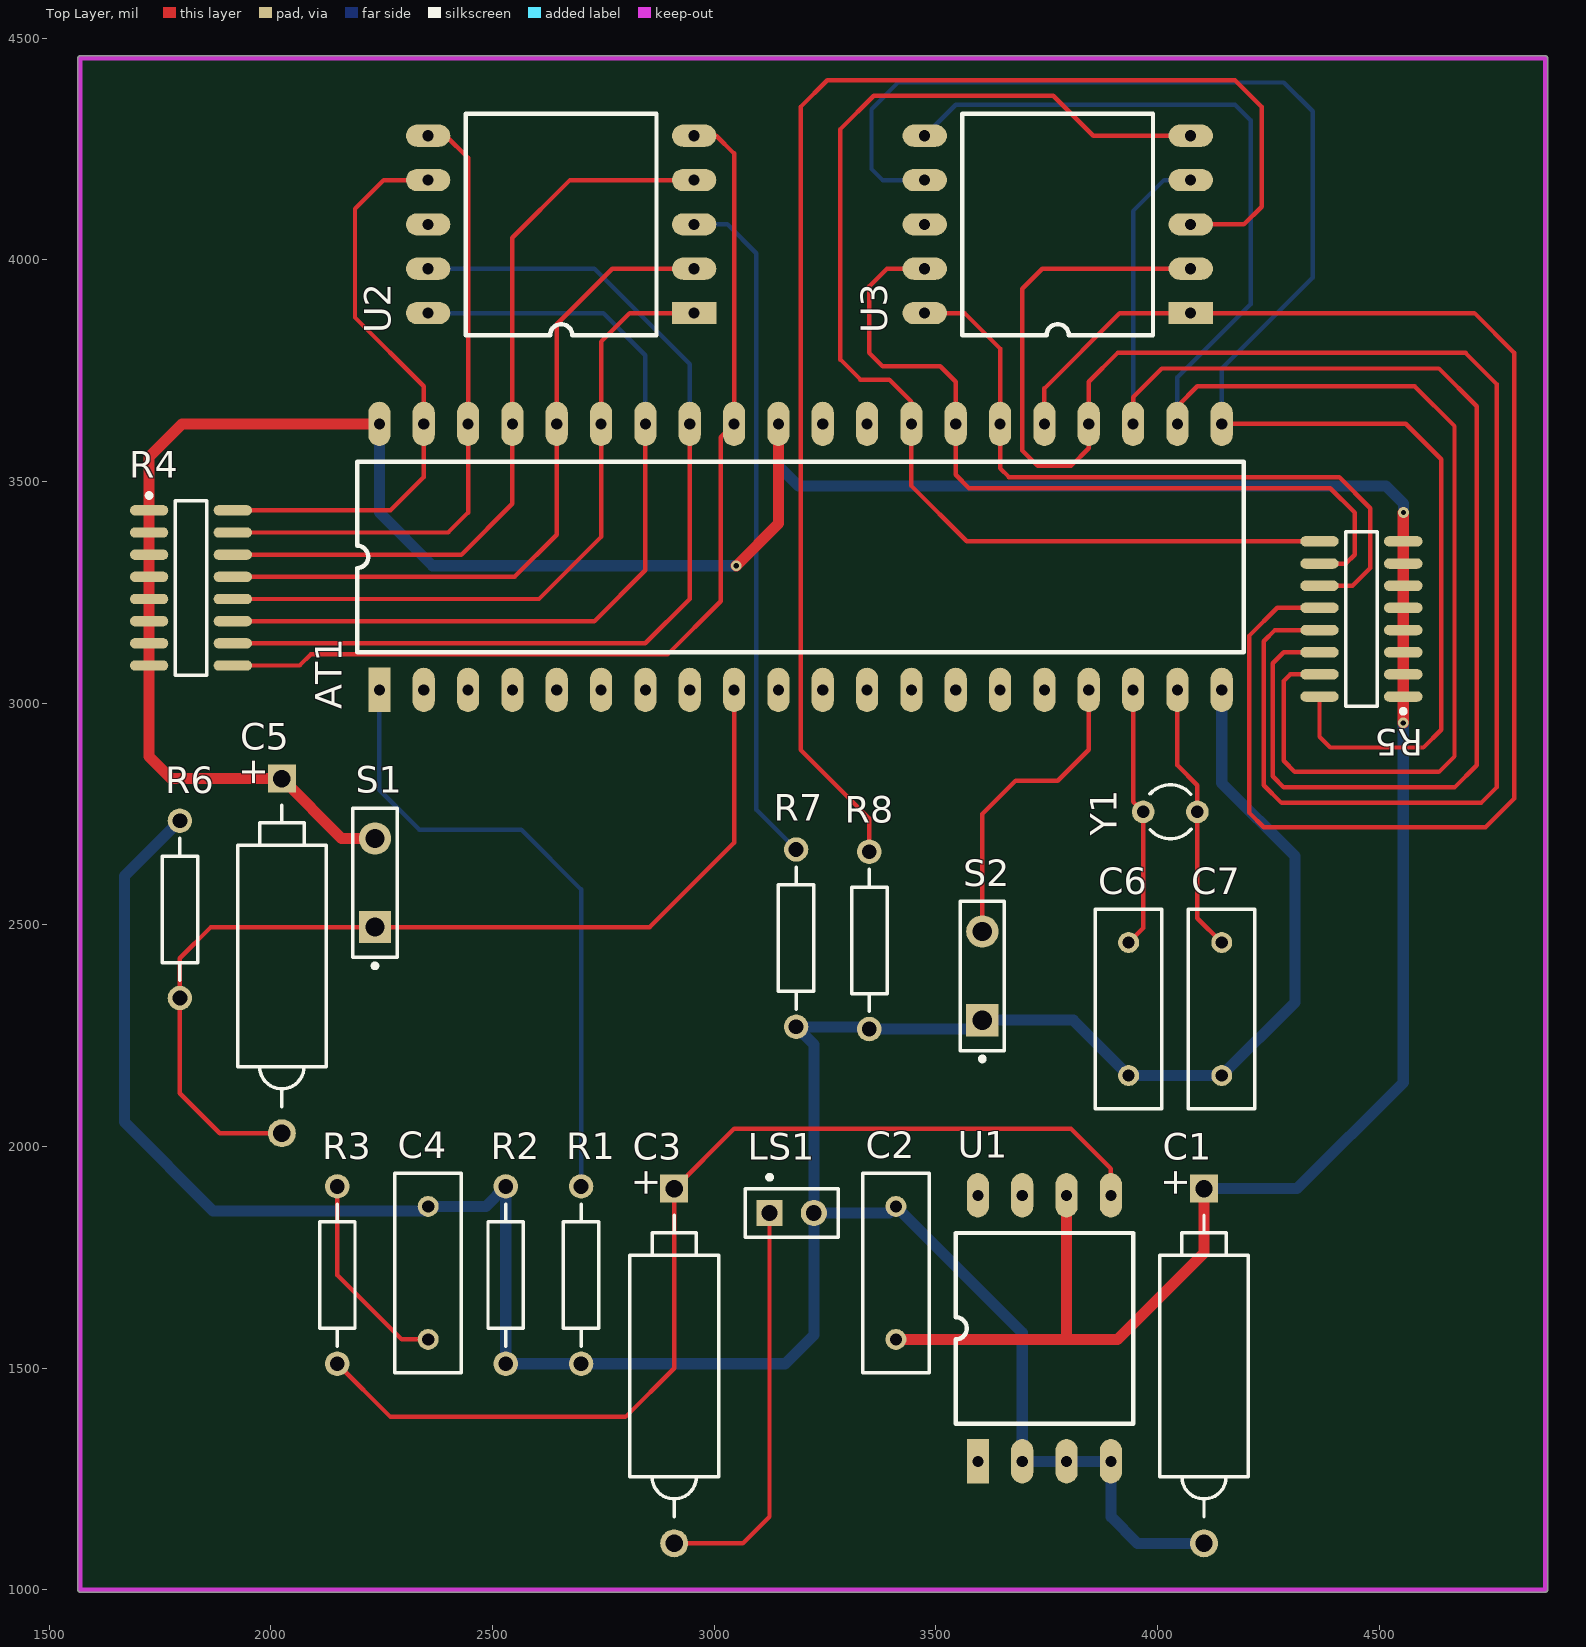
[diagram p0: Top Layer view]
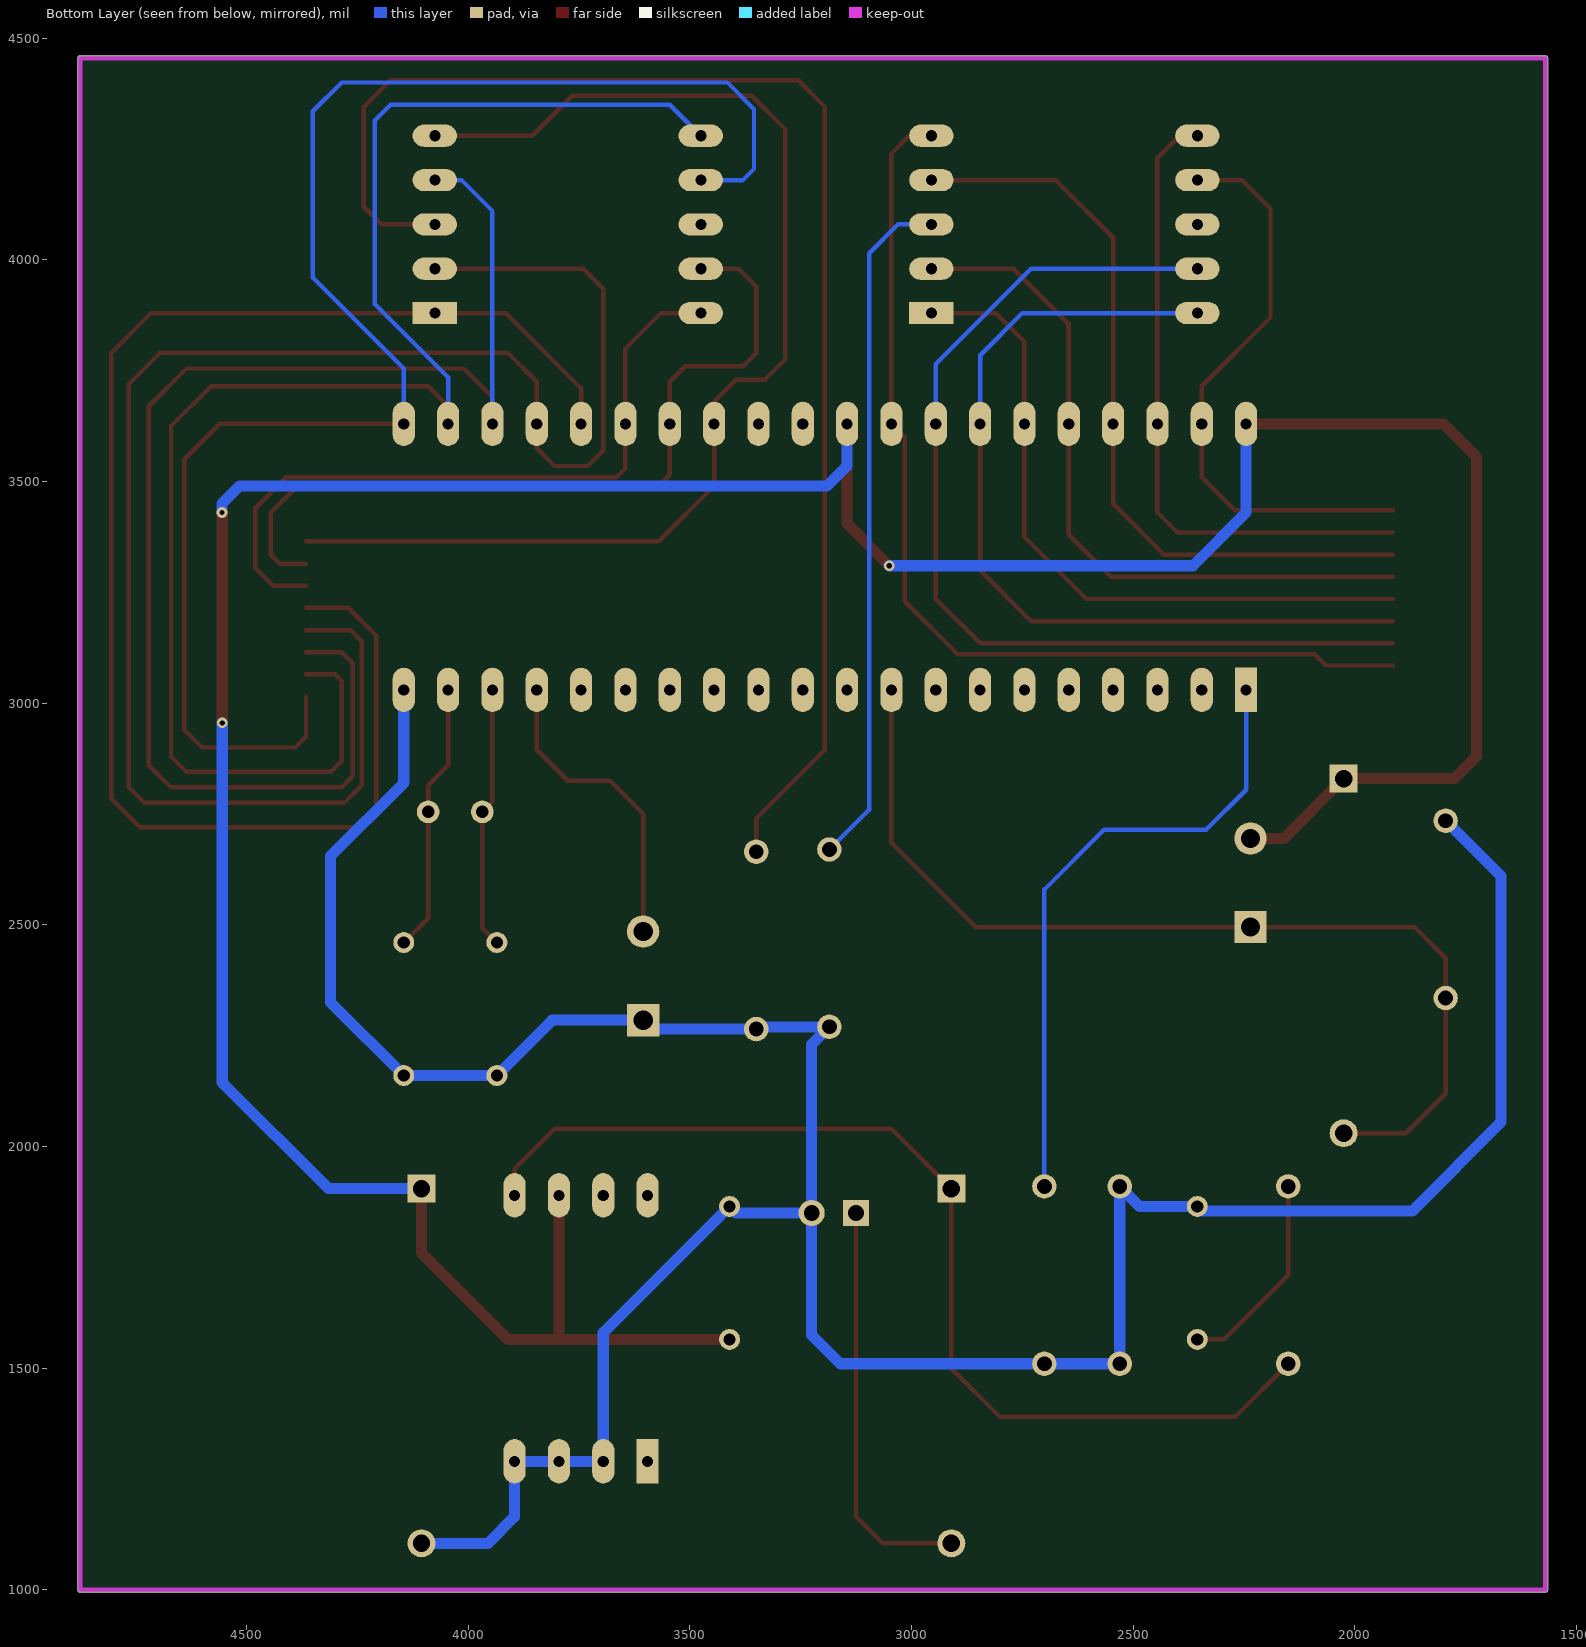
[diagram p1: Bottom Layer view, seen from below]
# Altium PCB MISC82805.PcbDoc
Units mil, origin at the board's own origin, x right, y up, seen from the top; angles counter-clockwise.
Board outline 3315.03 x 3465.03 mil, 2 copper layers (Top Layer, Bottom Layer); 23 components, 28 nets, 134 pads, 3 vias.

## Layer stack, top to bottom (the 12.6 mil dielectric is the usual default, probably not edited)
Top Solder: solder mask 0.4, Solder Resist, Dk 3.5
Top Layer: signal copper 1.4
Dielectric 1: dielectric 12.6, FR-4, Dk 4.8
Bottom Layer: signal copper 1.4
Bottom Solder: solder mask 0.4, Solder Resist, Dk 3.5

## Board outline
1564.98,1000 ccw(c1570,1000) 1570,994.99 4875,994.99 ccw(c4875,1000) 4880.02,1000 4880.02,4455 ccw(c4875,4455) 4875,4460.02 1570,4460.02 ccw(c1570,4455) 1564.98,4455

## Design rules (kind name [scope] priority, off if disabled: settings)
Clearance [All] p1: gap=10
MinimumSolderMaskSliver [All] p1: minsoldermaskwidth=0
PolygonConnect [All] p1: connectstyle=Relief reliefconductorwidth=10 reliefentries=4 polygonreliefangle="90 Angle" airgapwidth=10
RoutingVias [All] p1: holewidth=28 width=50 viastyle="Through Hole" minholewidth=28 minwidth=50 maxholewidth=28 maxwidth=50
SilkToSilkClearance [All] p1: silktosilkclearance=0
SilkToSolderMaskClearance [IsPad] p1: minsilkscreentomaskgap=0 clearancetoexposedcopper=TRUE
SolderMaskExpansion [All] p1: expansion=4
Width [All] p1: maxlimit=30 minlimit=10 preferedwidth=10
27 further rules are at their usual default settings.

## Components (designator, comment, footprint, x,y, rotation, side; value= is the part's Value field where it differs from the comment)
AT1 "U?" AT89S52 2245,3030 r90 top
C1 "10UF" POLAR0.8 4105,1505 r90 top
C2 "0.1UF" RAD-0.3 3410,1715 r90 top
C3 "47UF" POLAR0.8 2910,1505 r90 top
C4 "0.047UF" RAD-0.3 2355,1715 r90 top
C5 "10UF" POLAR0.8 2025,2430 r90 top
C6 "30PF" RAD-0.3 3935,2310 r90 top
C7 "30PF" RAD-0.3 4145,2310 r90 top
LS1 "Speaker" PIN2 3125,1850 r0 top
R1 "10K" AXIAL-0.4 2700,1710 r90 top
R2 "470" AXIAL-0.4 2530,1710 r90 top
R3 "47" AXIAL-0.4 2150,1710 r90 top
R4 "Res Pack3" SO-16_N 1820,3260 r0 top
R5 "Res Pack3" SO-16_N 4460,3190 r180 top
R6 "10K" AXIAL-0.4 1795,2535 r90 top
R7 "10K" AXIAL-0.4 3185,2470 r270 top
R8 "10K" AXIAL-0.4 3350,2465 r270 top
S1 "SW-PB" SPST-2 2235,2595 r90 top
S2 "SW-PB" SPST-2 3605,2385 r90 top
U1 "LM386N-1" LM386N-1 3595,1290 r90 top
U2 "LED8" LED8 2955,3880 r180 top
U3 "LED8" LED8 4075,3880 r180 top
Y1 "XTAL" R38 4028.98,2755 r90 top

## Footprints (in the part's own frame and the unit in brackets; to place one, negate y for a bottom-side part, rotate by r counter-clockwise, add the part's x,y. Pads: shape width x height; smd on the part's side, far side on the other; paste and mask are expansions set on the pad)
AT89S52 [mil]
  rect 100x50 hole 25: 1(0,0)
  oval 100x50 hole 25: 2(0,-100) 3(0,-200) 4(0,-300) 5(0,-400) 6(0,-500) 7(0,-600) 8(0,-700) 9(0,-800) 10(0,-900) 11(0,-1000) 12(0,-1100) 13(0,-1200) 14(0,-1300) 15(0,-1400) 16(0,-1500) 17(0,-1600) 18(0,-1700) 19(0,-1800) 20(0,-1900) 21(600,-1900) 22(600,-1800) 23(600,-1700) 24(600,-1600) 25(600,-1500) 26(600,-1400) 27(600,-1300) 28(600,-1200) 29(600,-1100) 30(600,-1000) 31(600,-900) 32(600,-800) 33(600,-700) 34(600,-600) 35(600,-500) 36(600,-400) 37(600,-300) 38(600,-200) 39(600,-100) 40(600,0)
  silkscreen extent 85,-1950 515,50
AXIAL-0.4 [mm] "Axial Device, Thru-Hole; 2 Leads; 0.4 in Pin Spacing"
  round 1.4 hole 0.85: 1(-5.08,0) 2(5.08,0)
  silkscreen extent -4.06,-1.02 4.06,1.02
LED8 [mil]
  rect 100x50 hole 25: 1(0,0)
  oval 100x50 hole 25: 2(0,-100) 3(0,-200) 4(0,-300) 5(0,-400) 6(600,-400) 7(600,-300) 8(600,-200) 9(600,-100) 10(600,0)
  silkscreen extent 85,-450 515,50
LM386N-1 [mil]
  rect 100x50 hole 25: 1(0,0)
  oval 100x50 hole 25: 2(0,-100) 3(0,-200) 4(0,-300) 5(600,-300) 6(600,-200) 7(600,-100) 8(600,0)
  silkscreen extent 85,-350 515,50
PIN2 [mm] "Photosensitive Diode; 2 Leads"
  rect 1.5x1.5 hole 0.9: 1(0,0)
  round 1.5 hole 0.9: 2(2.54,0)
  silkscreen extent -1.4,-1.4 3.94,2.17
POLAR0.8 [mm] "Polarized Capacitor; 2 Leads"
  rect 1.6x1.6 hole 1: 1(10.16,0)
  round 1.6 hole 1: 2(-10.16,0)
  silkscreen extent -8.64,-2.54 8.64,2.54
R38 [mm] "Crystal, Thru-Hole; 2 Leads; Body 3.1 x 8.2 mm (Dia.xH)"
  round 1.3 hole 0.7: 1(0,1.55) 2(0,-1.55)
  silkscreen extent -1.55,-1.19 1.55,1.17
RAD-0.3 [mm] "Radial Cap, Thru-Hole; 2 Leads; 0.3 in Pin Spacing"
  round 1.2 hole 0.7: 1(-3.81,0) 2(3.81,0)
  silkscreen extent -5.71,-1.91 5.71,1.91
SO-16_N [mm] "SOIC, 16-Leads, Body 9.9x3.9mm, Pitch 1.27mm, IPC Medium Density"
  oval 2.2x0.6 smd: 1(-2.4,4.445) 2(-2.4,3.175) 3(-2.4,1.905) 4(-2.4,0.635) 5(-2.4,-0.635) 6(-2.4,-1.905) 7(-2.4,-3.175) 8(-2.4,-4.445) 9(2.4,-4.445) 10(2.4,-3.175) 11(2.4,-1.905) 12(2.4,-0.635) 13(2.4,0.635) 14(2.4,1.905) 15(2.4,3.175) 16(2.4,4.445)
  silkscreen extent -2.52,-5 0.9,5.42, body extent -2,-5 2,5, height 1.75
SPST-2 [mm] "Switch; 2 Leads"
  rect 1.85x1.85 hole 1.1: 1(-2.54,0)
  round 1.85 hole 1.1: 2(2.54,0)
  silkscreen extent -4.89,-1.27 4.28,1.27

## Part data
AT1: library part AT89S52
C1 C3 C5: library part "Cap Pol2", "Polarized Capacitor (Axial)"
C2 C4 C6 C7: library part Cap, "Capacitor"
LS1: "Loudspeaker"
R1 R2 R3 R6 R7 R8: library part Res2, "Resistor"
R4 R5: "Isolated Resistor Network"
S1 S2: "Switch"
Y1: "Crystal Oscillator"

## Via types
v1: diameter 24, hole 12, Top Layer to Bottom Layer, 3 vias

## Nets (pads, with @x,y where several pads share a name; then routed paths per layer and width w, separated by ;. In a path a pad name is that pad's centre, name@x,y a point inside that pad or via, vN(x,y) a via of type N, cw(c..) or ccw(c..) an arc to the next point about the centre after c; other vN are vias at no path point)
GND: AT1.20 C1.2 C2.2 C4.2 C6.1 C7.1 LS1.2 R1.1 R2.1 R2.2 R6.2 R7.2 R8.2 S2.1 U1.2 U1.3 U1.4 | length 7013.8
  Bottom Layer w25: R6.2 1670,2610 1670,2055 1870,1855 2345,1855 C4.2 2485,1865 R2.2 R2.1 R1.1 3160,1510 3225,1575 LS1.2 ; C1.2 3955,1105 3895,1165 U1.4 U1.3 U1.2 3695,1580 C2.2 3395,1850 LS1.2 ; AT1.20 4145,2820 4310,2655 4310,2325 C7.1 C6.1 3810,2285 S2.1 3585,2265 R8.2 3355,2270 R7.2 3225,2230 LS1.2
NetAT1_1: AT1.1 R1.2 | length 1443.2
  Bottom Layer w10: AT1.1 2245,2805 2335,2715 2565,2715 2700,2580 R1.2
NetAT1_9: AT1.9 C5.2 R6.1 S1.1 | length 2275
  Top Layer w10: C5.2 1885,2030 1795,2120 R6.1 1795,2425 1865,2495 S1.1 2855,2495 3045,2685 AT1.9
NetAT1_17: AT1.17 S2.2 | length 700.1
  Top Layer w10: S2.2 3605,2750 3680,2825 3775,2825 3845,2895 AT1.17
NetAT1_18: AT1.18 C6.2 Y1.1 | length 593.2
  Top Layer w10: C6.2 3967.95,2492.95 Y1.1 3945,2777.95 AT1.18
NetAT1_19: AT1.19 C7.2 Y1.2 | length 611.4
  Top Layer w10: AT1.19 4045,2860 4090,2815 Y1.2 4090,2515 C7.2
NetC3_1: C3.1 R3.1 U1.5 | length 2398.5
  Top Layer w10: R3.1 2270,1390 2800,1390 2910,1500 C3.1 3045,2040 3805,2040 3895,1950 U1.5
NetC3_2: C3.2 LS1.1 | length 924.9
  Top Layer w10: C3.2 3065,1105 3125,1165 LS1.1
NetC4_1: C4.1 R3.2 | length 465.1
  Top Layer w10: R3.2 2150,1710 2295,1565 C4.1
NetR7_1: R7.1 U2.3 | length 1549.2
  Bottom Layer w10: U2.3 3030,4080 3095,4015 3095,2760 R7.1
NetR8_1: R8.1 U3.3 | length 3235.5
  Top Layer w10: R8.1 3350,2740 3195,2895 3195,4345 3255,4405 4175,4405 4235,4345 4235,4120 4195,4080 U3.3
P0.0: AT1.39 R4.16 U2.7 | length 1322.7
  Top Layer w10: R4.16 2270,3435 2345,3510 AT1.39 2345,3715 2190,3870 2190,4115 2255,4180 U2.7
P0.1: AT1.38 R4.15 U2.6 | length 1459.9
  Top Layer w10: R4.15 2400,3385 2445,3430 AT1.38 2445,4230 2395,4280 U2.6
P0.2: AT1.37 R4.14 U2.4 | length 1742
  Top Layer w10: R4.14 2430,3335 2545,3450 AT1.37 2545,4050 2675,4180 U2.4
P0.3: AT1.36 R4.13 U2.2 | length 1606.6
  Top Layer w10: R4.13 2550,3285 2645,3380 AT1.36 2645,3855 2770,3980 U2.2
P0.4: AT1.35 R4.12 U2.1 | length 1565.4
  Top Layer w10: R4.12 2605,3235 2745,3375 AT1.35 2745,3815 2810,3880 U2.1
P0.5: AT1.34 R4.11 U2.10 | length 1992.5
  Top Layer w10: R4.11 2730,3185 2845,3300 AT1.34
  Bottom Layer w10: U2.10 2750,3880 2845,3785 AT1.34
P0.6: AT1.33 R4.10 U2.9 | length 2281
  Top Layer w10: R4.10 2845,3135 2945,3235 AT1.33
  Bottom Layer w10: U2.9 2730,3980 2945,3765 AT1.33
P0.7: AT1.32 R4.9 U2.5 | length 2289.6
  Top Layer w10: R4.9 2065,3085 2090,3110 2895,3110 3015,3230 3015,3600 AT1.32 3045,4240 3005,4280 U2.5
P2.0: AT1.21 R5.16 U3.7 | length 3631.9
  Top Layer w10: AT1.21 4560,3630 4640,3550 4640,2940 4600,2900 4390,2900 4365.51,2924.49 R5.16
  Bottom Layer w10: U3.7 3380,4180 3355,4205 3355,4340 3415,4400 4285,4400 4350,4335 4350,3960 4145,3755 AT1.21
P2.1: AT1.22 R5.15 U3.6 | length 3674.3
  Top Layer w10: AT1.22 4045,3670 4090,3715 4580,3715 4670,3625 4670,2880 4635,2845 4310,2845 4285,2870 4285,3050 4300,3065 R5.15
  Bottom Layer w10: U3.6 3545,4350 4175,4350 4210,4315 4210,3900 4045,3735 AT1.22
P2.2: AT1.23 R5.14 U3.4 | length 3208.1
  Top Layer w10: AT1.23 3945,3690 4010,3755 4635,3755 4720,3670 4720,2860 4670,2810 4285,2810 4260,2835 4260,3090 4285,3115 R5.14
  Bottom Layer w10: AT1.23 3945,4110 4015,4180 U3.4
P2.3: AT1.24 R5.13 U3.2 | length 3997.6
  Top Layer w10: U3.2 3740,3980 3695,3935 3695,3570 3730,3535 3805,3535 3845,3575 AT1.24 3845,3725 3910,3790 4695,3790 4765,3720 4765,2810 4730,2775 4280,2775 4240,2815 4240,3140 4265,3165 R5.13
P2.4: AT1.25 R5.12 U3.1 | length 3474.5
  Top Layer w10: AT1.25 3745,3710 3915,3880 U3.1 4715,3880 4805,3790 4805,2785 4740,2720 4240,2720 4207.5,2752.5 4207.5,3152.5 4270,3215 R5.12
P2.5: AT1.26 R5.11 U3.10 | length 1611.5
  Top Layer w10: U3.10 3565,3880 3645,3800 AT1.26 3645,3530 3665,3510 4410,3510 4480,3440 4480,3305 4440,3265 R5.11
P2.6: AT1.27 R5.10 U3.9 | length 1841.5
  Top Layer w10: U3.9 3390,3980 3350,3940 3350,3790 3380,3760 3510,3760 3545,3725 AT1.27 3545,3515 3575,3485 4390,3485 4445,3430 4445,3335 4425,3315 R5.10
P2.7: AT1.28 R5.9 U3.5 | length 2740
  Top Layer w10: U3.5 3855,4280 3765,4370 3360,4370 3285,4295 3285,3775 3330,3730 3395,3730 3445,3680 AT1.28 3445,3490 3570,3365 R5.9
VCC: AT1.31 AT1.40 C1.1 C2.1 C5.1 R4.1 R4.2 R4.3 R4.4 R4.5 R4.6 R4.7 R4.8 R5.1 R5.2 R5.3 R5.4 R5.5 R5.6 R5.7 R5.8 S1.2 U1.6 | length 7869.5
  Top Layer w25: S1.2 2160,2695 C5.1 1775,2830 1725.51,2879.49 R4.8 R4.7 R4.6 R4.5 R4.4 R4.3 R4.2 R4.1 1725.51,3555.51 1800,3630 AT1.40 ; v1(3050,3310) 3145,3405 AT1.31 ; C2.1 3790,1565 ; U1.6 3795,1570 3790,1565 ; C1.1 4105,1760 3910,1565 3790,1565 ; v1@4555,2955 v1(4554.49,2955.51) R5.1 R5.2 R5.3 R5.4 R5.5 R5.6 R5.7 R5.8 4554.49,3429.49 v1(4555,3430)
  Bottom Layer w25: AT1.40 2245,3430 2365,3310 v1(3050,3310) ; AT1.31 3145,3535 3190,3490 4515,3490 4555,3450 v1(4555,3430) ; C1.1 4315,1905 4554.49,2144.49 v1(4554.49,2955.51)
pads on no net: AT1.2 AT1.3 AT1.4 AT1.5 AT1.6 AT1.7 AT1.8 AT1.10 AT1.11 AT1.12 AT1.13 AT1.14 AT1.15 AT1.16 AT1.29 AT1.30 U1.1 U1.7 U1.8 U2.8 U3.8

## Keep-outs
Keep-Out Layer:
  lines w10: 1570,4345 1570,4455 4875,4455 4875,1000 1595,1000 1570,1000 1570,4355